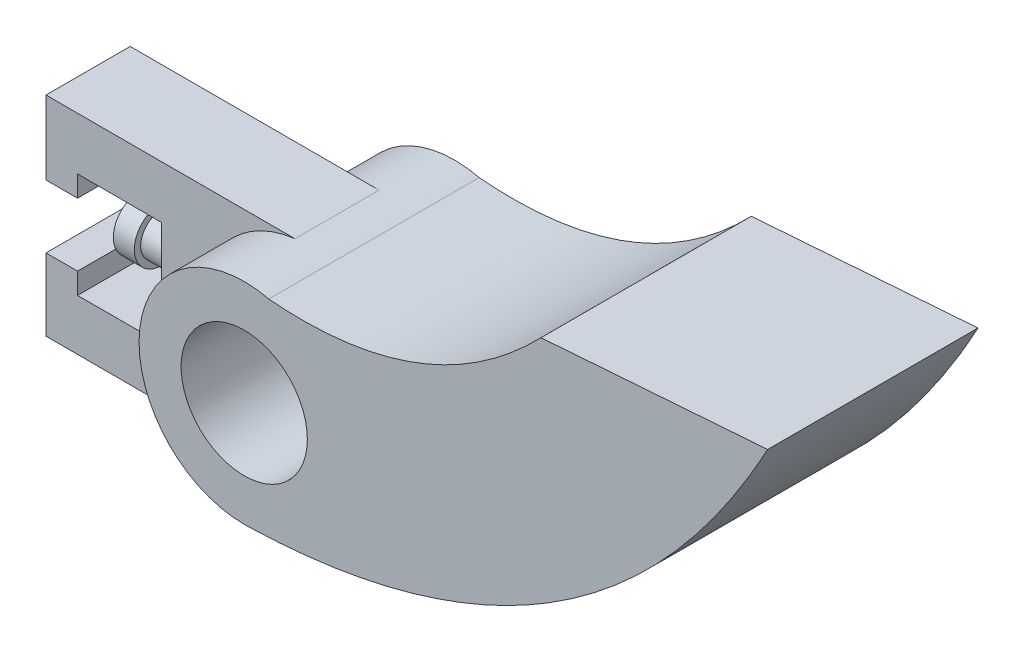
SolidWorks part; units mm, degrees
ref_plane "Front Plane" through (0, 0, 0) normal (0, 0, 1) x (1, 0, 0)
ref_plane "Top Plane" through (0, 0, 0) normal (0, 1, 0) x (1, 0, 0)
ref_plane "Right Plane" through (0, 0, 0) normal (1, 0, 0) x (0, 0, -1)
sketch "Sketch1" plane through (0, 0, 0) normal (0, 0, 1) x (1, 0, 0)
  circle A0 centre (0, 0) radius 3
  circle A1 centre (0, 0) radius 5
  dimension "D1" = 6
  dimension "D2" = 10
extrude "Boss-Extrude1" add sketch "Sketch1" along normal blind 10
sketch "Sketch2" plane through (0, 0, 10) normal (0, 0, 1) x (1, 0, 0)
  line L0 (24.8805, 10.5255) -> (14.1048, 9.7381)
  circle A0 centre (0, 0) radius 5 construction
  arc A1 (0, 5) -> (0, -5) centre (0, 0) ccw
  circle A2 centre (0, 0) radius 3
  spline S0 degree 2 poles (14.1048, 9.7381) (8.3234, 3.7698) (0, 5) knots 0 0 0 1 1 1
  spline S1 degree 2 poles (24.8805, 10.5255) (16.6899, -4.6319) (0, -5) knots 0 0 0 1 1 1
extrude "Boss-Extrude2" add sketch "Sketch2" against normal blind 10
sketch "Sketch3" plane through (0, 0, 10) normal (0, 0, 1) x (1, 0, 0)
  line L0 (-20.4234, -4.9652) -> (0, -4.9652)
  line L1 (-20.4234, -4.9652) -> (-20.4234, 4.9652)
  line L2 (0, -4.9652) -> (0, -3)
  line L3 (-20.4234, 4.9652) -> (0, 4.9652)
  line L4 (-20.4234, -4.9652) -> (0, 4.9652) construction
  line L5 (0, -4.9652) -> (-20.4234, 4.9652) construction
  line L6 (0, 3) -> (0, 4.9652)
  arc A0 (0, 3) -> (0, -3) centre (0, 0) ccw
  point P1 (-10.2117, 0)
extrude "Boss-Extrude3" add sketch "Sketch3" against normal blind 4 from offset 3 offset against normal yes
sketch "Sketch4" plane through (-20.4234, 0, 0) normal (-1, 0, 0) x (0, 0, 1)
  line L1 (3, 4.9652) -> (7, 4.9652)
  line L2 (3, 4.9652) -> (3, -4.9652)
  line L3 (3, -4.9652) -> (7, -4.9652)
  line L4 (7, 4.9652) -> (7, -4.9652)
extrude "Cut-Extrude1" cut sketch "Sketch4" against normal blind 8
sketch "Sketch6" plane through (0, 0, 7) normal (0, 0, 1) x (1, 0, 0)
  line L0 (-0.589, 4.9652) -> (-12.4234, 4.9652) construction
  line L1 (-12.4234, -4.9652) -> (-12.4234, 4.9652) construction
  line L2 (-12.4234, 1.4652) -> (-10.9234, 1.4652)
  line L3 (-10.9234, 1.4652) -> (-10.9234, 2.4652)
  line L4 (-10.9234, 2.4652) -> (-6.9234, 2.4652)
  line L5 (-6.9234, 2.4652) -> (-6.9234, -2.5348)
  line L6 (-6.9234, -2.5348) -> (-10.9234, -2.5348)
  line L7 (-10.9234, -2.5348) -> (-10.9234, -1.5348)
  line L8 (-10.9234, -1.5348) -> (-12.4234, -1.5348)
  line L9 (-12.4234, -1.5348) -> (-12.4234, 1.4652)
  dimension "D1" = 1.5
  dimension "D2" = 4
  dimension "D3" = 1
  dimension "D4" = 1.5
  dimension "D5" = 1
  dimension "D6" = 5
  dimension "D7" = 2.5
extrude "Cut-Extrude3" cut sketch "Sketch6" against normal blind 6
sketch "Sketch7" plane through (-6.9234, 0, 0) normal (-1, 0, 0) x (0, 0, 1)
  circle A0 centre (5, 0) radius 1
  dimension "D1" = 2
extrude "Boss-Extrude4" add sketch "Sketch7" along normal blind 3
sketch "Sketch8" plane through (-9.9234, 0, 0) normal (-1, 0, 0) x (0, 0, 1)
  circle A0 centre (5, 0) radius 1.3
  dimension "D1" = 2.6
extrude "Boss-Extrude5" add sketch "Sketch8" against normal blind 1
